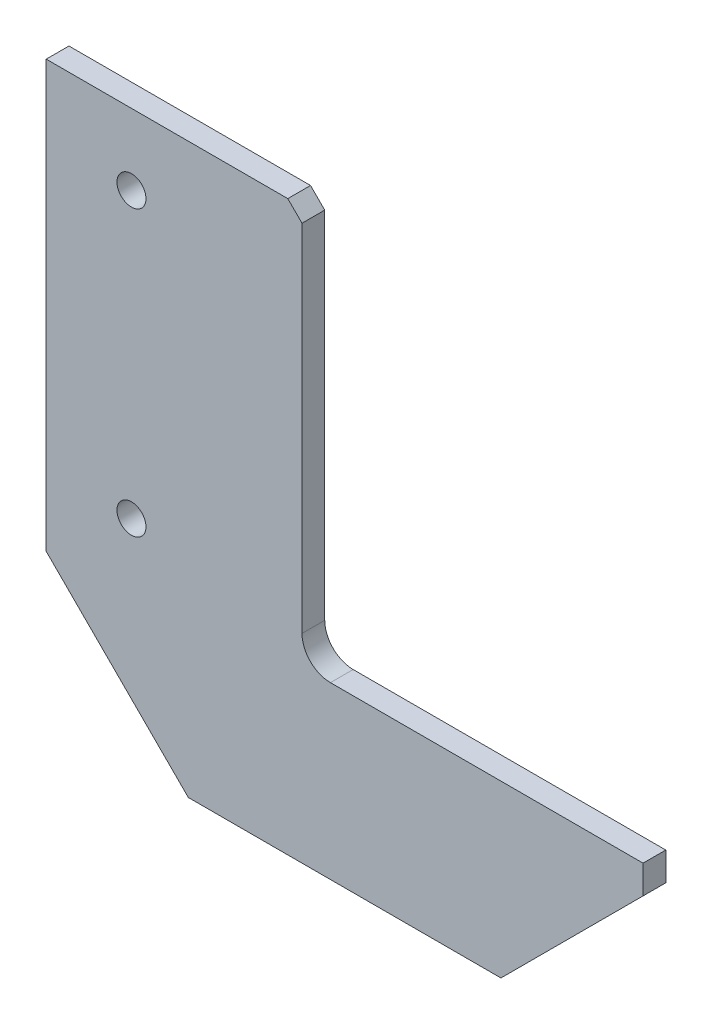
from build123d import *

# Parameters (mm, degrees)
SKETCH1_W              = 210
SKETCH1_H              = 200
BOSS_EXTRUDE1_DEPTH    = 8
CHAMFER1_SIZE          = 50
M12_TAPPED_HOLE1_D     = 10.2
M12_TAPPED_HOLE1_DEPTH = 29.25
M12_TAPPED_HOLE1_TIP   = 3.064389157
SKETCH5_W              = 180.548294757
SKETCH5_H              = 165.829683772
CUT_EXTRUDE1_DEPTH     = 8
CHAMFER2_SIZE          = 5
FILLET1_R              = 10


with BuildPart() as part:
    # Sketch1 → Boss-Extrude1 (new body)
    with BuildSketch(Plane.XY):
        Rectangle(SKETCH1_W, SKETCH1_H)
    extrude(amount=BOSS_EXTRUDE1_DEPTH)

    # Chamfer1
    chamfer1_edges = [part.edges().sort_by_distance(p)[0] for p in [
        (105, -100, 4),
        (-105, -100, 4),
    ]]
    chamfer(chamfer1_edges, length=CHAMFER1_SIZE)

    # M12 Tapped Hole1
    with Locations(Plane.XY.offset(8)):
        with Locations((-75, 75.01), (-75, -24.99)):
            Hole(M12_TAPPED_HOLE1_D / 2, depth=M12_TAPPED_HOLE1_DEPTH)
            with Locations((0, 0, -(M12_TAPPED_HOLE1_DEPTH + M12_TAPPED_HOLE1_TIP / 2))):  # 118° drill point
                Cone(0, M12_TAPPED_HOLE1_D / 2, M12_TAPPED_HOLE1_TIP, mode=Mode.SUBTRACT)

    # Sketch5 → Cut-Extrude1 (cut)
    with BuildSketch(Plane.XY.offset(8)):
        with Locations((75.274147379, 42.914841886)):
            Rectangle(SKETCH5_W, SKETCH5_H)
    extrude(amount=-CUT_EXTRUDE1_DEPTH, mode=Mode.SUBTRACT)

    # Chamfer2
    chamfer2_edges = [part.edges().sort_by_distance(p)[0] for p in [
        (-15, 100, 4),
    ]]
    chamfer(chamfer2_edges, length=CHAMFER2_SIZE)

    # Fillet1
    fillet1_edges = [part.edges().sort_by_distance(p)[0] for p in [
        (-15, -40, 4),
    ]]
    fillet(fillet1_edges, radius=FILLET1_R)


solid = part.part
